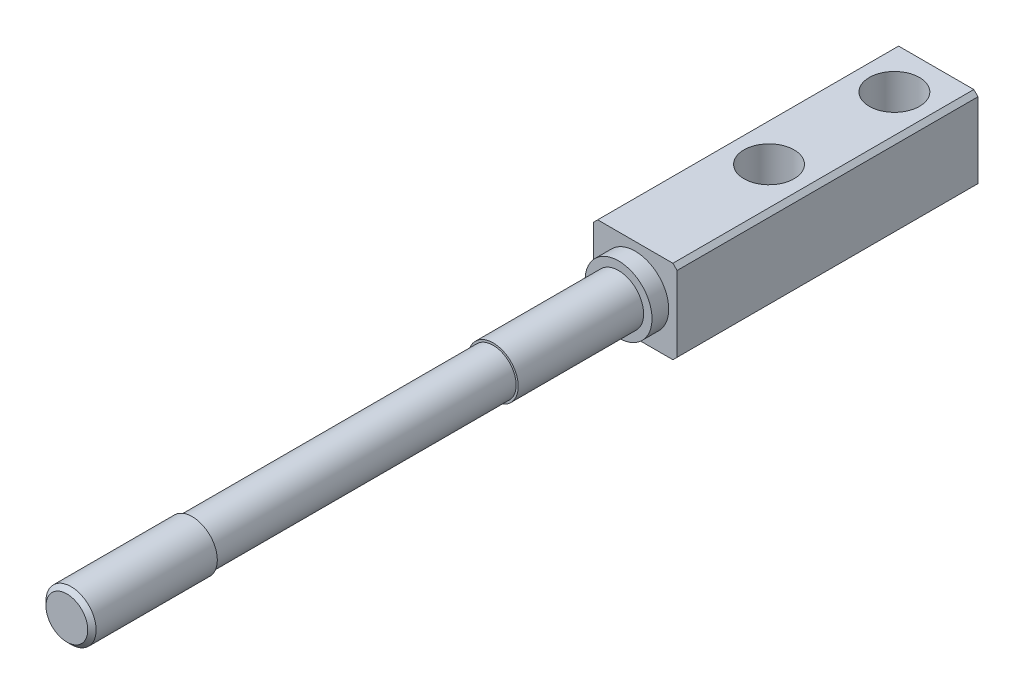
SolidWorks part; units mm, degrees
ref_plane "Front Plane" through (0, 0, 0) normal (0, 0, 1) x (1, 0, 0)
ref_plane "Top Plane" through (0, 0, 0) normal (0, 1, 0) x (1, 0, 0)
ref_plane "Right Plane" through (0, 0, 0) normal (1, 0, 0) x (0, 0, -1)
sketch "Sketch1" plane through (0, 0, 0) normal (0, 0, 1) x (1, 0, 0)
  line L1 (-5, 5) -> (5, 5)
  line L2 (-5, 5) -> (-5, -5)
  line L3 (-5, -5) -> (5, -5)
  line L4 (5, 5) -> (5, -5)
  line L5 (-5, 5) -> (5, -5) construction
  line L6 (-5, -5) -> (5, 5) construction
  point P0 (0, 0)
  dimension "D1" = 10
  dimension "D2" = 10
extrude "Boss-Extrude1" add sketch "Sketch1" along normal blind 36
sketch "Sketch2" plane through (0, 0, 36) normal (0, 0, 1) x (1, 0, 0)
  circle A0 centre (0, 0) radius 4
  dimension "D1" = 8
extrude "Boss-Extrude2" add sketch "Sketch2" along normal blind 2
sketch "Sketch3" plane through (0, 0, 38) normal (0, 0, 1) x (1, 0, 0)
  circle A0 centre (0, 0) radius 3
  dimension "D1" = 6
extrude "Boss-Extrude3" add sketch "Sketch3" along normal blind 66
sketch "Sketch4" plane through (0, 5, 0) normal (0, 1, 0) x (1, 0, 0)
  line L0 (5, -36) -> (-5, -36) construction
  circle A0 centre (0, -5) radius 3
  circle A1 centre (0, -20) radius 3
  dimension "D3" = 6
  dimension "D1" = 16
  dimension "D2" = 15
extrude "Cut-Extrude1" cut sketch "Sketch4" against normal blind 50
chamfer "Chamfer1" distance 0.5 angle 45 4 edges at (5, -5, 18) (5, 5, 18) (-5, 5, 18) (-5, -5, 18)
chamfer "Chamfer2" distance 0.5 angle 45 1 edges at (3, 0, 104)
sketch "Sketch6" plane through (0, 0, 0) normal (0, 1, 0) x (1, 0, 0)
  line L0 (-3, -38) -> (3, -38) construction
  line L1 (2.75, -53) -> (7.75, -53)
  line L2 (2.75, -53) -> (2.75, -89)
  line L3 (2.75, -89) -> (7.75, -89)
  line L4 (7.75, -53) -> (7.75, -89)
  line L5 (-2.5, -104) -> (2.5, -104) construction
  line L6 (3, -103.5) -> (3, -38) construction
  dimension "D1" = 15
  dimension "D2" = 15
  dimension "D3" = 0.25
  dimension "D4" = 5
ref_axis "Axis1" through (0, 0, 103.5) along (0, 0, -1)
revolve "Cut-Revolve1" cut sketch "Sketch6" angle 360 about axis through (0, 0, 103.5) along (0, 0, -1)
